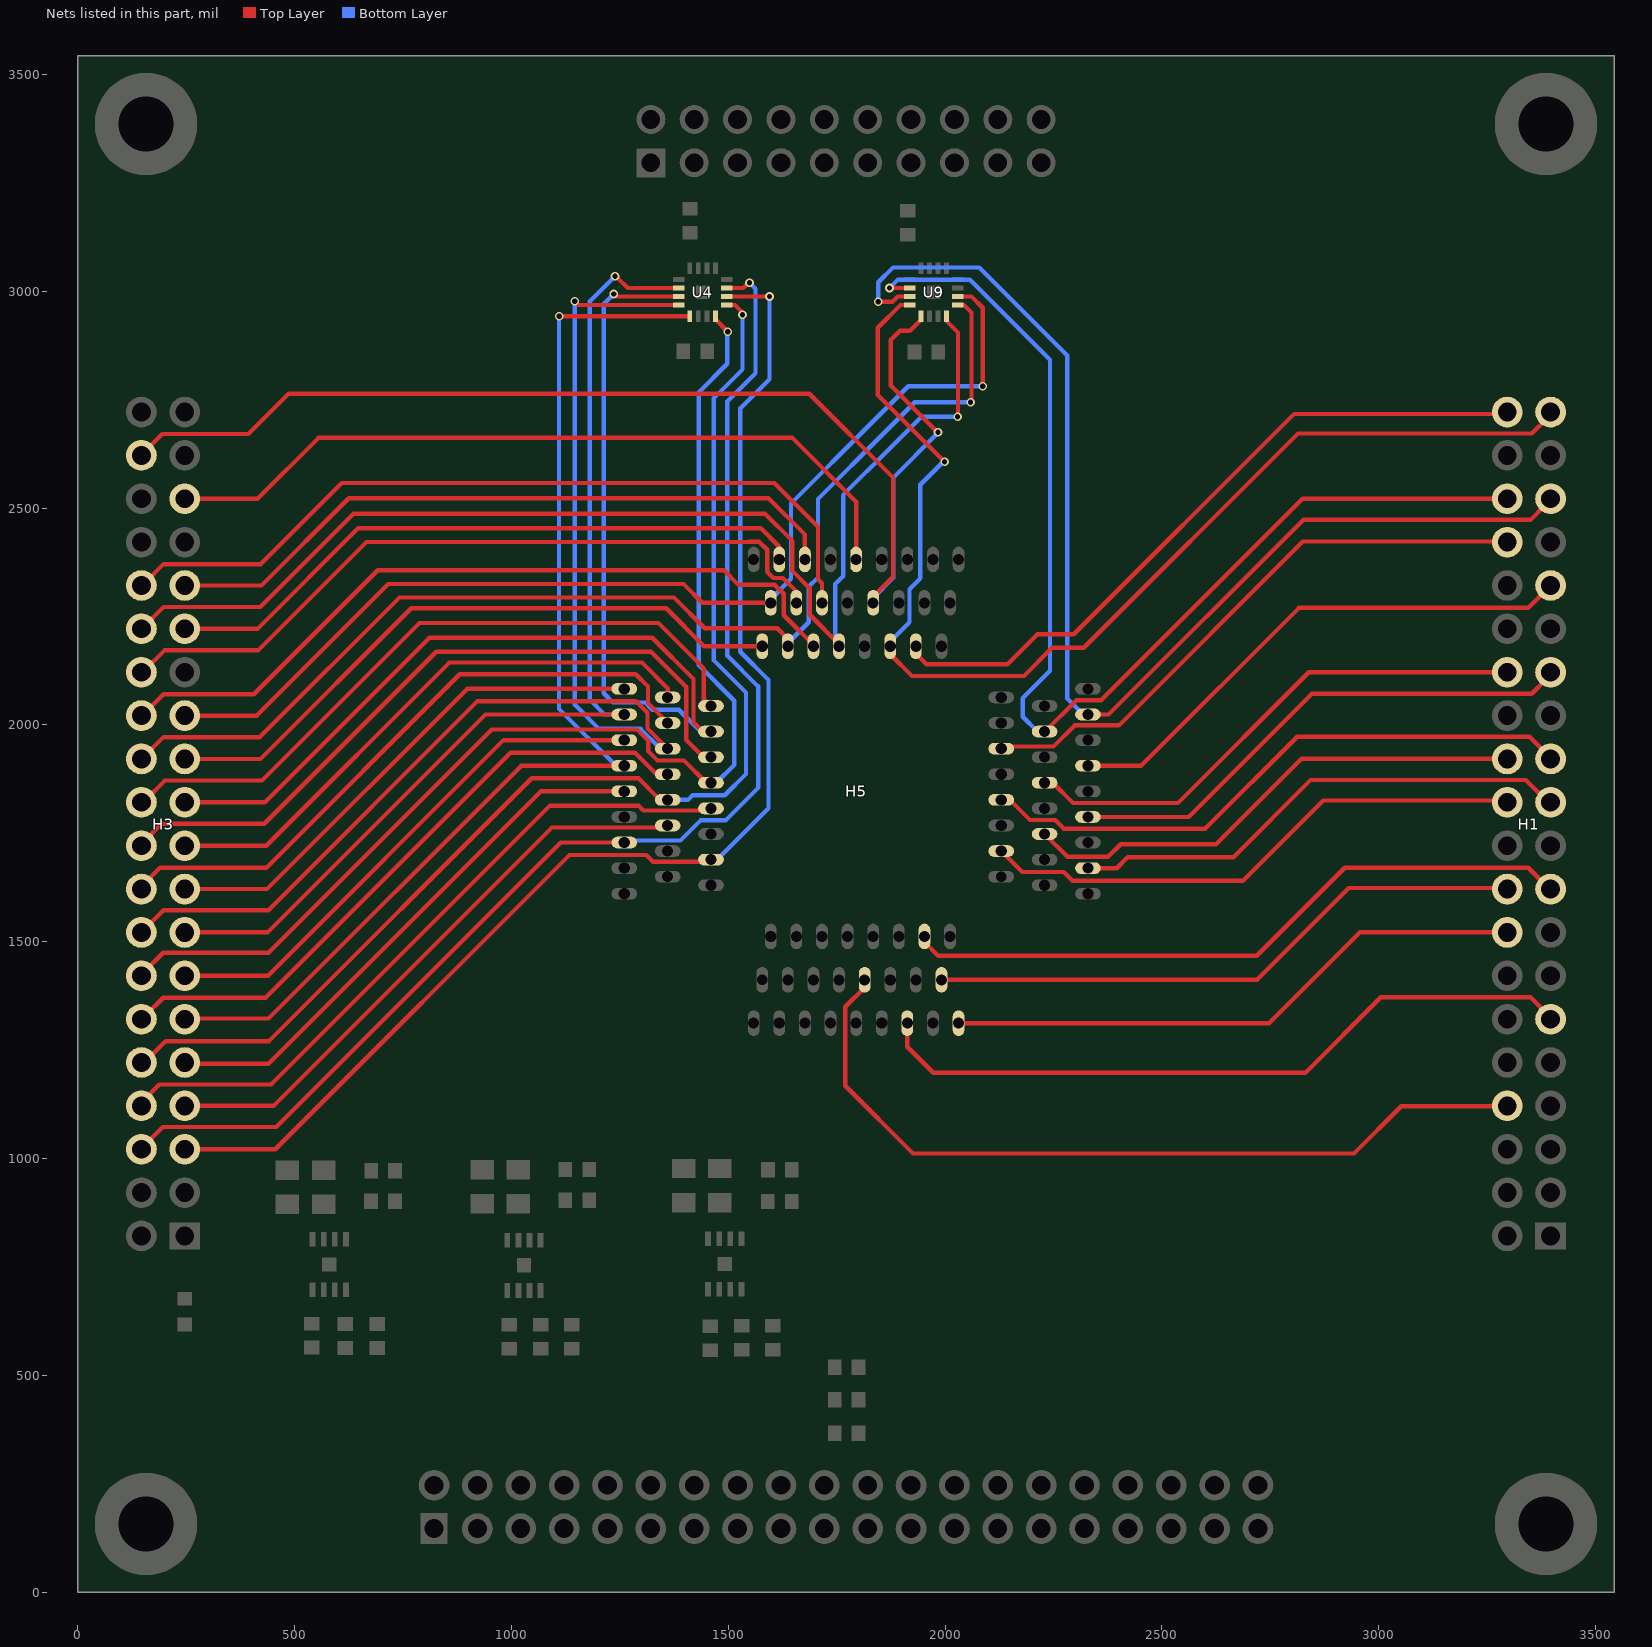
[diagram p0: the nets of this part, all layers, seen from the top]
# Altium PCB MISC62795.pcbdoc (part 2 of 2)
Units mil, origin at the board's own origin, x right, y up, seen from the top; angles counter-clockwise.
Board outline 3543.31 x 3543.31 mil, 4 copper layers (Top Layer, GND, POWER, Bottom Layer); 39 components, 94 nets, 363 pads, 705 vias.

## Via types
v1: diameter 20, hole 12, Top Layer to Bottom Layer, 705 vias

## Nets (pads, with @x,y where several pads share a name; then routed paths per layer and width w, separated by ;. In a path a pad name is that pad's centre, name@x,y a point inside that pad or via, vN(x,y) a via of type N, cw(c..) or ccw(c..) an arc to the next point about the centre after c; other vN are vias at no path point) (continued)
OTA_BIAS: H1.36 H5.45 U9.2 | length 2703.9
  Top Layer w10: v1(1872.16,3007.84) U9.2@1918.59,3007.84 ; H5.45@2229.65,1984.8 2230.8,1984.8 2303,2057 2360,2057 2824.65,2521.65 H1.36@3296.46,2521.65
  Bottom Layer w10: v1(1872.16,3007.84) 1891.31,3027 2057,3027 2242,2842 2242,2125 2179,2062 2179,2019 2213.2,1984.8 H5.45@2229.65,1984.8
RST: H3.19 H5.77 | length 1334.1
  Top Layer w10: H3.19@246.85,1721.65 434.65,1721.65 857,2144 1301,2144 1360.35,2084.65 H5.77@1360.35,2063.54
RST16_1: H1.40 H5.56 | length 1675.7
  Top Layer w10: H5.56@1932.8,2181.65 1932.8,2164.2 1957,2140 2144,2140 2213,2209 2297,2209 2805,2717 3192,2717 ; 3245,2717 3192,2717 ; H1.40@3289,2717 3192,2717
S0: H1.21 H5.29 | length 1157.1
  Top Layer w10: H5.29@2329.65,1669.83 2395.83,1669.83 2421,1695 2665,1695 2843,1873 3339,1873 H1.21@3384,1828
S1: H1.22 H5.31 | length 1298.5
  Top Layer w10: H5.31@2129.65,1709.2 2177.85,1661 2274,1661 2294,1641 2687,1641 2872,1826 3231,1826 ; 3244,1826 3231,1826 ; H1.22@3307,1818 3299,1826 3231,1826
S2: H1.24 H5.33 | length 1174.2
  Top Layer w10: H5.33@2229.65,1748.57 2282.22,1696 2376,1696 2405,1725 2625,1725 2822,1922 3191,1922 ; 3200,1922 3191,1922 ; H1.24@3279,1921 3278,1922 3191,1922
S_IN0: H1.16 H5.25 | length 1362.9
  Top Layer w10: H5.25@2031.22,1312.35 2747.35,1312.35 2957,1522 3226,1522 ; 3242,1522 3226,1522 ; H1.16@3290,1519 3287,1522 3226,1522
S_IN1: H1.18 H5.23 | length 1417.1
  Top Layer w10: H5.23@1991.85,1412.35 2719.35,1412.35 2931,1624 3216,1624 ; 3243,1624 3216,1624 ; H1.18@3293,1621 3290,1624 3216,1624
S_IN2: H1.8 H5.14 | length 1934.6
  Top Layer w10: H5.14@1814.68,1412.35 1814.68,1394.68 1770,1350 1770,1168 1926,1012 2943,1012 3052,1121 3203,1121 ; 3244,1121 3203,1121 ; H1.8@3291,1121 3203,1121
S_IN3: H1.17 H5.21 | length 1570.4
  Top Layer w10: H5.21@1952.48,1512.35 1952.48,1499.52 1984,1468 2719,1468 2922,1671 3345,1671 H1.17@3393,1623
S_IN4: H1.11 H5.19 | length 1642
  Top Layer w10: H5.19@1913.11,1312.35 1913.11,1257.89 1973,1198 2831,1198 3005,1372 3350,1372 H1.11@3388,1334
SAMPLE: H3.35 H5.63 | length 1800.5
  Top Layer w10: H3.35@246.85,2521.65 414.65,2521.65 555,2662 1648,2662 1795,2515 H5.63@1795,2381.65
SL_OFF_CHIP: H1.34 H5.43 | length 1357.2
  Top Layer w10: H5.43@2129.65,1945.43 2134.46,1950.24 2250.24,1950.24 2299,1999 2401,1999 2825,2423 H1.34@3289,2423
V_GP0_0: H1.23 H5.37 | length 1393
  Top Layer w10: H5.37@2129.65,1827.32 2149.68,1827.32 2196,1781 2254,1781 2274,1761 2600,1761 2812,1973 3348,1973 H1.23@3390,1931
V_GP0_1: H1.31 H5.41 | length 1229.7
  Top Layer w10: H5.41@2329.65,1906.06 2452.06,1906.06 2816,2270 3345,2270 H1.31@3390,2315
V_GP1_0: H1.27 H5.35 | length 1187.7
  Top Layer w10: H5.35@2329.65,1787.95 2561.95,1787.95 2846,2072 3353,2072 H1.27@3386,2105
V_GP1_1: H1.28 H5.39 | length 1211.1
  Top Layer w10: H5.39@2229.65,1866.69 2248.31,1866.69 2295,1820 2537,1820 2838.65,2121.65 H1.28@3296.46,2121.65
VBCAP: H3.24 H5.71 U9.9 | length 2785.4
  Top Layer w10: H3.24@151,1925 198,1972 420,1972 742,2294 1375,2294 1446,2223 1613,2223 1637.52,2198.48 H5.71@1637.52,2181.65 ; U9.9@2029.41,2968.47 2043.53,2968.47 2061,2951 2061,2782 ; v1@2058,2741 2061,2744 2061,2782 ; 2061,2762 2061,2782
  Bottom Layer w10: H5.71@1637.52,2181.65 1637.52,2188.52 1686,2237 1686,2319 1707,2340 1707,2521 1860,2674 ; 1865,2679 1860,2674 ; v1(2059,2744) 1930,2744 1860,2674
VBCLEAR: H3.30 H5.65 U9.8 | length 2951.3
  Top Layer w10: H3.30@155,2229 198,2272 421,2272 636,2487 801,2487 ; 722,2487 801,2487 ; H5.65@1755.63,2181.65 1755.63,2186.37 1688,2254 1688,2315 1648,2355 1648,2424 1585,2487 801,2487 ; U9.8@2003.53,2942.59 2003.53,2931.47 2030,2905 2030,2804 ; v1@2028,2709 2030,2711 2030,2804 ; 2030,2794 2030,2804
  Bottom Layer w10: H5.65@1755.63,2181.65 1747,2190.28 1747,2325 1765,2343 1765,2530 1872.5,2637.5 ; 1876.5,2641.5 1872.5,2637.5 ; v1(2029,2711) 1946,2711 1872.5,2637.5
VBCOMP: H3.25 H5.73 U9.10 | length 2545.9
  Top Layer w10: H3.25@246.85,2021.65 412.65,2021.65 716,2325 1397,2325 1440.35,2281.65 H5.73@1598.15,2281.65 ; U9.10@2029.41,2988.16 2060.84,2988.16 2087,2962 v1@2087,2782
  Bottom Layer w10: H5.73@1598.15,2281.65 1598.15,2290.15 1645,2337 1645,2511 1832,2698 1915,2781 v1(2087,2781)
VBIASN: H1.39 H5.59 U9.4 | length 2848.4
  Top Layer w10: 1845,2772 1845,2874 ; H5.59@1873.74,2181.65 1873.74,2163.26 1924,2113 2182,2113 2247,2178 2320,2178 2814,2672 3353,2672 H1.39@3389,2708 ; U9.4@1918.59,2968.47 1897.47,2968.47 1845,2916 1845,2874 ; v1(1999,2607) 1845,2761 1845,2874
  Bottom Layer w10: H5.59@1873.74,2181.65 1873.74,2192.74 1917.93,2236.93 1917.93,2312.93 1943,2338 1943,2554 v1@1997,2608
VBIASP: H3.38 H5.61 U9.5 | length 2994.2
  Top Layer w10: H3.38@157,2633 195,2671 393,2671 486,2764 1687,2764 1880,2571 1880,2342 1834.37,2296.37 H5.61@1834.37,2281.65 ; 1875,2799 1875,2818 ; U9.5@1944,2934 1919,2909 1896,2909 1875,2888 1875,2818 ; U9.5@1944.47,2934 U9.5@1944.47,2942.59 ; v1(1984,2675) 1984,2674 1875,2783 1875,2818
  Bottom Layer w10: H5.61@1834.37,2281.65 1834.37,2293.37 1881,2340 1881,2571 v1@1983,2673
VBN: H3.21 H5.81 U4.3 | length 2925.9
  Top Layer w10: H3.21@246.85,1821.65 431.65,1821.65 811,2201 1325,2201 1419.83,2106.17 1419.83,2006.17 1441.2,1984.8 H5.81@1460.35,1984.8 ; v1(1236,2994) 1241.84,2988.16 U4.3@1385.59,2988.16
  Bottom Layer w10: 1213,2951 1213,2933 ; v1@1235,2993 1213,2971 1213,2933 ; 1240.9,2052 1265,2052 ; H5.81@1460.35,1984.8 1436.2,1984.8 1386,2035 1325,2035 1308,2052 1265,2052 ; 1213,2933 1213,2073 1234,2052 1265,2052
VBP: H3.15 H5.79 U4.2 | length 2503.2
  Top Layer w10: H3.15@246.85,1521.65 437.65,1521.65 940.17,2024.17 H5.79@1260.35,2024.17 ; v1@1245,3031 1268.16,3007.84 U4.2@1385.59,3007.84
  Bottom Layer w10: 1181,2948 1181,2911 ; v1(1239,3035) 1181,2977 1181,2911 ; H5.79@1260.35,2024.17 1214.83,2024.17 1181,2058 1181,2911
VCLAMP: H1.35 H5.47 U9.3 | length 2762.2
  Top Layer w10: v1(1846,2976) 1879,2976 1891.16,2988.16 U9.3@1918.59,2988.16 ; H5.47@2329.65,2024.17 2377.17,2024.17 2826,2473 3350,2473 H1.35@3382,2505
  Bottom Layer w10: v1(1846,2976) 1846,3021 1880,3055 2079,3055 2282,2852 2282,2061 2318.83,2024.17 H5.47@2329.65,2024.17
VCLEAR: H3.32 H5.67 | length 1894.5
  Top Layer w10: H3.32@157,2330 198,2371 422,2371 609,2558 754,2558 ; 725,2558 754,2558 ; H5.67@1716.26,2281.65 1716.26,2326.74 1707,2336 1707,2457 1606,2558 754,2558
VDELAY_N: H3.11 H5.85 U4.5 | length 2670.7
  Top Layer w10: H3.11@246.85,1321.65 H3.11@262,1321.65 ; H3.11@262,1323 440,1323 1023.06,1906.06 H5.85@1260.35,1906.06 ; v1(1110.41,2942.59) U4.5@1411.47,2942.59
  Bottom Layer w10: v1@1110,2947 1110,2037 1240.94,1906.06 H5.85@1260.35,1906.06
VDELAY_P: H3.16 H5.83 U4.4 | length 2934
  Top Layer w10: H3.16@155,1530 198,1573 440,1573 922,2055 1287,2055 1314,2028 1314,1991.78 H5.83@1360.35,1945.43 ; v1(1146,2977) 1154.53,2968.47 U4.4@1385.59,2968.47
  Bottom Layer w10: 1146,2948 1146,2933 ; v1(1146,2977) 1146,2933 ; H5.83@1360.35,1945.43 1343.57,1945.43 1298,1991 1202,1991 1146,2047 1146,2933
VEN: H3.31 H5.69 | length 1677.7
  Top Layer w10: H3.31@246.85,2321.65 423.65,2321.65 625,2523 792,2523 ; 720,2523 792,2523 ; H5.69@1676.89,2381.65 1676.89,2439.11 1593,2523 792,2523
VREFN: H3.10 H5.89 U4.9 | length 2854.9
  Top Layer w10: H3.10@165,1233 203,1271 441,1271 1047,1877 1293,1877 1342.68,1827.32 H5.89@1360.35,1827.32 ; U4.9@1496.41,2968.47 1515.53,2968.47 v1@1533,2951
  Bottom Layer w10: H5.89@1360.35,1827.32 1407.32,1827.32 1418,1838 1492,1838 1541,1887 1541,2075 1467,2149 1467,2699 ; 1467,2705 1467,2699 ; v1(1533,2946) 1533,2820 1467,2754 1467,2699
VREFP: H3.14 H5.87 U4.8 | length 2778.7
  Top Layer w10: H3.14@154,1432 197,1475 440,1475 954.61,1989.61 1289.39,1989.61 1316,1963 1316,1939 1337,1918 1398,1918 1449.31,1866.69 H5.87@1460.35,1866.69 ; U4.8@1470.53,2942.59 1470.53,2935.47 v1(1499,2907)
  Bottom Layer w10: H5.87@1460.35,1866.69 1472.69,1866.69 1514,1908 1514,2056 1432,2138 1432,2767 1498,2833 v1@1498,2905
WL_IN0: H3.5 H5.96 U4.10 | length 3018.2
  Top Layer w10: H3.5@246.85,1021.65 455.65,1021.65 1134,1700 1311,1700 1326.3,1684.7 1455.54,1684.7 H5.96@1460.35,1689.52 ; U4.10@1496.41,2988.16 v1(1595.16,2988.16)
  Bottom Layer w10: H5.96@1460.35,1689.52 1474.52,1689.52 1593,1808 1593,2104 1528,2169 1528,2730 1595.16,2797.16 v1(1595.16,2988.16)
WL_IN1: H3.6 H5.94 U4.11 | length 3034.8
  Top Layer w10: H3.6@156,1033 196,1073 458,1073 1113.89,1728.89 H5.94@1260.35,1728.89 ; U4.11@1496.41,3007.84 1534.84,3007.84 v1@1546,3019
  Bottom Layer w10: H5.94@1260.35,1728.89 1265.17,1733.7 1389.7,1733.7 1436,1780 1494,1780 1569,1855 1569,2089 1498,2160 1498,2746 1563,2811 1563,3006 v1(1549,3020)
Y0: H3.7 H5.92 | length 1381.3
  Top Layer w10: H3.7@246.85,1121.65 451.65,1121.65 1093.45,1763.45 1355.54,1763.45 H5.92@1360.35,1768.26
Y1: H3.8 H5.90 | length 1593.4
  Top Layer w10: H3.8@154,1137 188,1171 446,1171 1089,1814 1293,1814 1304.18,1802.82 1455.54,1802.82 H5.90@1460.35,1807.63
Y2: H3.9 H5.88 | length 1352.3
  Top Layer w10: H3.9@266,1217 268,1219 396,1219 ; 299,1219 396,1219 ; H5.88@1260.35,1847 1068,1847 440,1219 396,1219
Y3: H3.12 H5.86 | length 1474.5
  Top Layer w10: H3.12@157,1331 197,1371 433,1371 998,1936 1285,1936 1334.63,1886.37 H5.86@1360.35,1886.37
Y4: H3.20 H5.84 | length 1657.8
  Top Layer w10: H3.20@155,1734 193,1772 430,1772 827,2169 1322,2169 1403,2088 1403,1966 1443.26,1925.74 H5.84@1460.35,1925.74
Y5: H3.13 H5.82 | length 1238.6
  Top Layer w10: H3.13@246.85,1421.65 438.65,1421.65 982.11,1965.11 H5.82@1260.35,1965.11
Y6: H3.18 H5.80 | length 1474.1
  Top Layer w10: H3.18@155,1636 190,1671 435,1671 881,2117 1287,2117 1315,2089 1315,2051 1360.35,2005.65 H5.80@1360.35,2004.48
Y7: H3.22 H5.78 | length 1589.2
  Top Layer w10: H3.22@159,1830 201,1872 425,1872 788,2235 1339,2235 1444,2130 1444,2060.2 H5.78@1460.35,2043.85
Y8: H3.17 H5.76 | length 1204.7
  Top Layer w10: H3.17@246.85,1621.65 436.65,1621.65 898.22,2083.22 H5.76@1260.35,2083.22
Y9: H3.23 H5.74 | length 1511.7
  Top Layer w10: H3.23@246.85,1921.65 421.65,1921.65 769,2269 1357,2269 1444.35,2181.65 H5.74@1578.46,2181.65
Y10: H3.29 H5.72 | length 1618.5
  Top Layer w10: H3.29@246.85,2221.65 414.65,2221.65 647,2454 827,2454 ; 723,2454 827,2454 ; H5.72@1617.83,2381.65 1617.83,2411.17 1575,2454 827,2454
Y11: H3.28 H5.70 | length 1809.6
  Top Layer w10: H3.28@158,2130 200,2172 256,2172 416,2172 666,2422 805,2422 ; 719,2422 805,2422 ; H5.70@1657.2,2281.65 1657.2,2307.8 1626,2339 1604,2339 1590,2353 1590,2404 1571.83,2422.17 1548.63,2422.17 1548.46,2422 805,2422
Y12: H3.26 H5.68 | length 1934.3
  Top Layer w10: H3.26@157,2030 198,2071 406,2071 692,2357 879,2357 ; 723,2357 879,2357 ; H5.68@1696.57,2181.65 1696.57,2184.43 1628,2253 1628,2302.47 1607.47,2323 1524,2323 1490,2357 879,2357
pads on no net: H2.2 H5.1 H5.2 H5.4 H5.6 H5.8 H5.10 H5.12 H5.49 H5.50 H5.51 H5.52 H5.53 H5.95 H5.97 H5.98 H5.99 H5.100

## Polygon pours and split planes (outlines as drawn)
GND on Top Layer "Bottom Layer-No Net" (solid, remove dead copper): -240,3599 -240,-65 -79,-226 24,-329 393,-329 3632,-329 3783,-178 3943,-18 3943,275 3943,3589 3754,3778 3622,3910 3603,3910 72,3910 -230,3608
DVDDIO on Top Layer "Bottom Layer-No Net" (solid, remove dead copper): 1786,250 1786,75 1798,63 1806,55 1841,55 2759,55 2767,63 2774,70 2776,72 2776,476 2776,550 2762,564 2743,583 2449,583 1805,583 1790,568 1786,564 1786,250
DVDD on Top Layer "Bottom Layer-No Net" (solid, remove dead copper): 1498,833 1498,800 1499,799 1502,799 1598,799 1599,800 1608,809 1608,899 1608,1001 1603,1006 1598,1011 1584,1011 1461,1011 1455,1005 1452,1002 1452,988 1452,962 1458,956 1459,955 1473,955 1510,955 1518,947 1521,944 1521,936 1521,875 1508,862 1498,852 1498,834
5.0V on Top Layer "Bottom Layer-No Net" (solid, remove dead copper, pour order 1000): 98,820 98,770 98,687 118,667 126,659 226,659 299,659 306,666 315,675 315,695 315,839 305,849 301,853 286,853 120,853 107,840 99,832 99,823
5V on Top Layer "Bottom Layer-No Net" (solid, remove dead copper, pour order 1001): 101,619 101,510 109,502 112,499 158,499 292,499 310,517 314,521 314,562 314,609 295,628 289,634 256,634 116,634 102,620
5V on Top Layer "Bottom Layer-No Net" (solid, remove dead copper, pour order 1002): 586,698 586,683 586,616 599,603 600,602 605,602 728,602 733,607 738,612 738,619 738,696 726,708 719,715 626,715 589,715 587,713 586,712 586,698
DVDDIO on Top Layer "Bottom Layer-No Net" (solid, remove dead copper, pour order 1003): 585,833 585,800 586,799 587,798 590,798 675,798 677,800 692,815 692,886 692,1004 685,1011 679,1017 651,1017 549,1017 542,1010 539,1007 539,986 539,959 543,955 545,953 560,953 599,953 602,950 609,943 609,925 609,874 599,864 585,850 585,833
5V on Top Layer "Bottom Layer-No Net" (solid, remove dead copper, pour order 1004): 1035,700 1035,608 1045,598 1109,598 1161,598 1166,603 1172,609 1172,616 1172,688 1161,699 1147,713 1076,713 1041,713 1038,710 1035,707 1035,700
AVDD on Top Layer "Bottom Layer-No Net" (solid, remove dead copper, pour order 1005): 1035,831 1035,799 1038,796 1039,795 1048,795 1118,795 1124,801 1141,818 1141,896 1141,999 1139,1001 1134,1006 1125,1006 996,1006 993,1003 990,1000 990,991 990,959 994,955 997,952 1015,952 1047,952 1053,946 1057,942 1057,933 1057,872 1047,862 1035,850 1035,831
5V on Top Layer "Bottom Layer-No Net" (solid, remove dead copper, pour order 1006): 1498,697 1498,614 1509,603 1513,599 1528,599 1624,599 1627,602 1630,605 1630,615 1630,692 1623,699 1607,715 1537,715 1505,715 1501,711 1498,708 1498,698
GND on Bottom Layer "Bottom Layer-No Net" (solid, remove dead copper): -282,3386 -189,3293 -189,-180 3678,-180 3747,-111 3862,4 3862,328 3862,3652 3758,3756 3585,3929 3227,3929 -28,3929 -155,3802 -258,3699 -258,3433
GND on GND (split plane): 3523.21,20.1 20.1,20.1 20.1,3523.21 3523.21,3523.21
DVDDIO on POWER (split plane): 3523.21,20.1 1785.09,20.1 1785.09,475.82 1885.13,575.87 1886.74,577.96 1887.74,580.39 1888.09,583 1888.09,844 1887.74,846.61 1886.74,849.04 1885.13,851.13 1860.76,875.5 2439.13,1453.87 2440.74,1455.96 2441.45,1457.68 2441.74,1458.39 2442.09,1461 2442.09,1615 2441.74,1617.61 2441.45,1618.32 2440.74,1620.04 2439.13,1622.13 2386.13,1675.13 2384.04,1676.74 2381.61,1677.74 2379,1678.09 2323,1678.09 2320.39,1677.74 2319.17,1677.24 2317.96,1676.74 2315.87,1675.13 2282.82,1642.09 2198.18,1642.09 2183.09,1657.18 2183.09,1775 2182.74,1777.61 2181.74,1780.04 2180.13,1782.13 2161.13,1801.13 2159.04,1802.74 2156.61,1803.74 2154,1804.09 1754.18,1804.09 1729.76,1828.5 2064.13,2162.87 2065.74,2164.96 2066.24,2166.17 2066.74,2167.39 2067.09,2170 2067.09,2348 2066.74,2350.61 2066.03,2352.33 2065.74,2353.04 2064.13,2355.13 1993.13,2426.13 1991.04,2427.74 1988.61,2428.74 1986,2429.09 1581,2429.09 1578.39,2428.74 1575.96,2427.74 1573.87,2426.13 842.87,1695.13 841.26,1693.04 840.26,1690.61 839.91,1688 839.91,942.17 839.87,942.13 814.82,917.09 498.18,917.09 483.09,932.18 483.09,1988.82 1266.18,2771.91 1923,2771.91 1925.61,2772.26 1928.04,2773.26 1930.13,2774.87 2047.13,2891.87 2048.74,2893.96 2049.03,2894.67 2049.74,2896.39 2050.09,2899 2050.09,3015 2049.74,3017.61 2049.03,3019.33 2048.74,3020.04 2047.13,3022.13 2005.13,3064.13 2003.04,3065.74 2000.61,3066.74 1998,3067.09 1386.18,3067.09 1317.09,3136.18 1317.09,3523.21 3523.21,3523.21
5V on POWER (split plane): 1296.91,3132 1297.26,3129.39 1298.26,3126.96 1299.87,3124.87 1374.87,3049.87 1376.96,3048.26 1379.39,3047.26 1382,3046.91 1993.82,3046.91 2029.91,3010.82 2029.91,2903.18 1918.82,2792.09 1262,2792.09 1259.39,2791.74 1256.96,2790.74 1254.87,2789.13 465.87,2000.13 464.27,1998.04 463.26,1995.61 462.91,1993 462.91,928 463.26,925.39 464.27,922.96 465.87,920.87 486.87,899.87 488.96,898.27 490.17,897.76 491.39,897.26 494,896.91 819,896.91 821.61,897.26 824.04,898.27 826.13,899.87 847.5,921.24 903.87,864.87 905.96,863.27 908.39,862.26 911,861.91 1245,861.91 1247.61,862.26 1250.04,863.27 1252.13,864.87 1314.5,927.24 1373.87,867.87 1375.96,866.27 1378.39,865.26 1381,864.91 1835.8,864.91 1837.39,864.26 1840,863.91 1843.82,863.91 1867.91,839.82 1867.91,587.18 1767.87,487.13 1766.26,485.04 1765.26,482.61 1764.91,480 1764.91,20.1 20.1,20.1 20.1,3523.21 1296.91,3523.21
AVDD on POWER (split plane): 2046.91,2343.82 2046.91,2174.18 1306.87,1434.13 1305.26,1432.04 1304.26,1429.61 1303.91,1427 1303.91,946.2 1303.26,944.61 1303.24,944.51 1240.82,882.09 915.18,882.09 860.91,936.36 860.74,937.61 860.09,939.2 860.09,1683.82 1585.18,2408.91 1981.82,2408.91
DVDD on POWER (split plane): 1742.87,1786.87 1744.96,1785.26 1747.39,1784.26 1750,1783.91 2149.82,1783.91 2162.91,1770.82 2162.91,1653 2163.26,1650.39 2164.26,1647.96 2165.87,1645.87 2186.87,1624.87 2188.96,1623.26 2190.17,1622.76 2191.39,1622.26 2194,1621.91 2287,1621.91 2289.61,1622.26 2292.04,1623.26 2294.13,1624.87 2327.18,1657.91 2374.82,1657.91 2421.91,1610.82 2421.91,1465.18 1841.82,885.09 1385.18,885.09 1324.09,946.18 1324.09,1422.82 1715.5,1814.24

## Keep-outs
Keep-Out Layer:
  the board outline again, w10

## Other copper
POWER (plane layer: these items are gaps in the copper):
  lines w20: 851,935 847,935 819,907 494,907 473,928 473,1993 1262,2782 1923,2782 2040,2899 2040,3015 1998,3057 1382,3057 1307,3132 1307,3532 ; 1313,942 1314,942 1381,875 1846,875 2432,1461 2432,1615 2379,1668 2323,1668 2287,1632 2194,1632 2173,1653 2173,1775 2154,1794 1750,1794 1717,1827 ; 1775,15 1775,480 1878,583 1878,844 1848,874 1840,874 ; 850,933 911,872 1245,872 1314,941 1314,1427 2057,2170 2057,2348 1986,2419 1581,2419 850,1688 850,933

## Silkscreen, mask and mechanical layers (free items; w line width, h text height)
Top Overlay:
  text "GND" at 2011,3507 h40
  text "DIN2" at 1694,3506 h40
  text "GND" at 1799,3505 h40
  text "DIN1" at 1891,3505 h40
  text "DCLK" at 2102,3504 h40
  text "NC" at 1279,3503 h40
  text "GND" at 1380,3503 h40
  text "ROUT2" at 1472,3503 h40
  text "GND" at 1596,3503 h40
  text "GND" at 2210,3503 h40
  text "GND" at 2013,3466 h40
  text "DOUT1" at 1890,3465 h40
  text "EN_LDO" at 1233,3463 h40
  text "GND" at 1798,3462 h40
  text "DEN" at 2108,3462 h40
  text "GND" at 1381,3461 h40
  text "GND" at 2208,3461 h40
  text "DOUT2" at 1468,3460 h40
  text "GND" at 1595,3460 h40
  text "ROUT1" at 1679,3460 h40
  text "RST16_1" at 2877,2707 h40
  text "CK" at 329,2706 h40
  text "EN_DEC" at 441,2705 h40
  text "VBIASN" at 3069,2704 h40
  text "VBIASP" at 323,2606 h40
  text "INST3" at 485,2606 h40
  text "EN_CON" at 3061,2605 h40
  text "EN_WL_MUX" at 2810,2604 h40
  text "SAMPLE" at 470,2511 h40
  text "INST2" at 320,2508 h40
  text "OTA_BIAS" at 2838,2508 h40
  text "VCLAMP" at 3056,2507 h40
  text "EN_SL_MUX" at 3020,2409 h40
  text "INST1" at 325,2406 h40
  text "INST0" at 473,2405 h40
  text "SL_OFF_CHIP" at 2759,2405 h40
  text "V_GP0_1" at 3066,2311 h40
  text "EN_BL_MUX" at 2818,2310 h40
  text "VCLEAR" at 311,2307 h40
  text "VEN" at 500,2303 h40
  text "DAT1" at 3122,2210 h40
  text "DAT0" at 2968,2208 h40
  text "Y10" at 516,2206 h40
  text "VBCLEAR" at 315,2204 h40
  text "Y11" at 326,2111 h40
  text "V_GP1_0" at 3077,2110 h40
  text "V_GP1_1" at 2888,2108 h40
  text "HEAD" at 449,2107 h40
  text "GND" at 3142,2010 h40
  text "GND" at 2965,2009 h40
  text "Y12" at 322,2008 h40
  text "VBCOMP" at 447,2008 h40
  text "VBCAP" at 329,1914 h40
  text "Y9" at 499,1914 h40
  text "V_GP0_0" at 3078,1908 h40
  text "S2" at 2989,1906 h40
  text "S0" at 3132,1810 h40
  text "Y7" at 316,1809 h40
  text "VBN" at 419,1808 h40
  text "S1" at 2989,1808 h40
  text "Y4" at 320,1709 h40
  text "MUX_EN" at 3089,1707 h40
  text "DAT2" at 2970,1706 h40
  text "RST" at 418,1705 h40
  text "Y6" at 327,1609 h40
  text "S_IN3" at 3132,1609 h40
  text "S_IN1" at 3002,1608 h40
  text "Y8" at 430,1606 h40
  text "VBP" at 536,1509 h40
  text "VDELAY_P" at 313,1507 h40
  text "S_IN0" at 3006,1504 h40
  text "DAT4" at 3140,1503 h40
  text "Y5" at 478,1410 h40
  text "VREFP" at 319,1409 h40
  text "DAT5" at 3006,1408 h40
  text "DAT3" at 3138,1408 h40
  text "Y3" at 329,1313 h40
  text "VDELAY_N" at 422,1313 h40
  text "S_IN4" at 3132,1305 h40
  text "ADDR6" at 2976,1303 h40
  text "Y2" at 464,1214 h40
  text "VREFN" at 315,1211 h40
  text "DAT6" at 3141,1209 h40
  text "ADDR5" at 2979,1208 h40
  text "Y1" at 316,1116 h40
  text "Y0" at 375,1116 h40
  text "S_IN2" at 2977,1106 h40
  text "ADDR4" at 3119,1106 h40
  text "ADDR3" at 3115,1010 h40
  text "ADDR1" at 2966,1008 h40
  text "WL_IN1" at 349,972 h40 r90
  text "WL_IN0" at 413,970 h40 r90
  text "ADDR2" at 3112,906 h40
  text "ADDR0" at 2962,905 h40
  text "GND" at 413,873 h40 r90
  text "GND" at 349,871 h40 r90
  text "5V" at 416,803 h40 r90
  text "5V" at 353,802 h40 r90
  text "DAT7" at 3116,802 h40
  text "GND" at 2979,801 h40
  text "DIO" at 2101,310 h40
  text "DIO" at 2203,310 h40
  text "DIO" at 1897,308 h40
  text "DIO" at 1998,308 h40
  text "DIO" at 1798,307 h40
  text "DIO" at 2303,307 h40
  text "DIO" at 2405,307 h40
  text "DIO" at 2500,307 h40
  text "DIO" at 2607,307 h40
  text "DIO" at 2709,307 h40
  text "GND" at 778,306 h40
  text "GND" at 885,306 h40
  text "GND" at 983,306 h40
  text "GND" at 1081,306 h40
  text "GND" at 1180,306 h40
  text "GND" at 1280,306 h40
  text "GND" at 1382,306 h40
  text "GND" at 1483,306 h40
  text "GND" at 1580,306 h40
  text "GND" at 1681,306 h40
  text "DIO" at 1791,49 h40
  text "DIO" at 1891,49 h40
  text "DIO" at 1991,49 h40
  text "DIO" at 2091,49 h40
  text "DIO" at 2192,49 h40
  text "DIO" at 2293,49 h40
  text "DIO" at 2395,49 h40
  text "DIO" at 2490,49 h40
  text "DIO" at 2597,49 h40
  text "DIO" at 2699,49 h40
  text "GND" at 778,48 h40
  text "GND" at 885,48 h40
  text "GND" at 983,48 h40
  text "GND" at 1081,48 h40
  text "GND" at 1180,48 h40
  text "GND" at 1280,48 h40
  text "GND" at 1382,48 h40
  text "GND" at 1483,48 h40
  text "GND" at 1580,48 h40
  text "GND" at 1681,48 h40